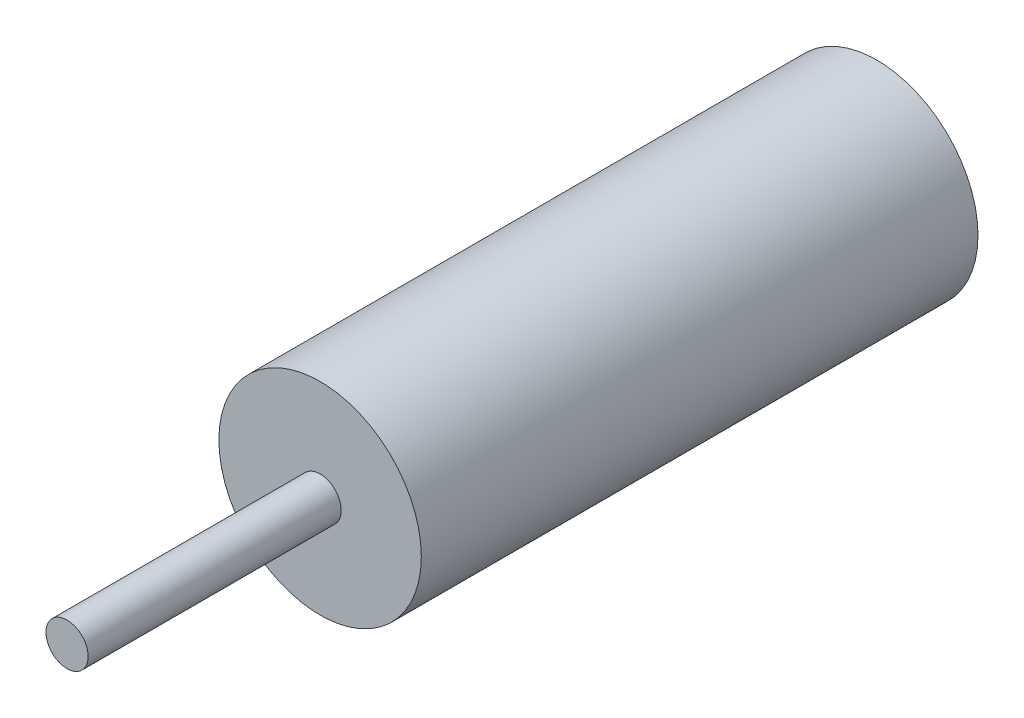
from build123d import *

# Parameters (mm, degrees)
SKETCH_1_R      = 6
EXTRUDE_1_DEPTH = 33
SKETCH_2_R      = 1.25
EXTRUDE_2_DEPTH = 15


with BuildPart() as part:
    # 草图1 → 凸台-拉伸1 (new body)
    with BuildSketch(Plane.XY):
        Circle(SKETCH_1_R)
    extrude(amount=EXTRUDE_1_DEPTH)

    # 草图2 → 凸台-拉伸2 (add)
    with BuildSketch(Plane.XY.offset(33)):
        Circle(SKETCH_2_R)
    extrude(amount=EXTRUDE_2_DEPTH)


solid = part.part
